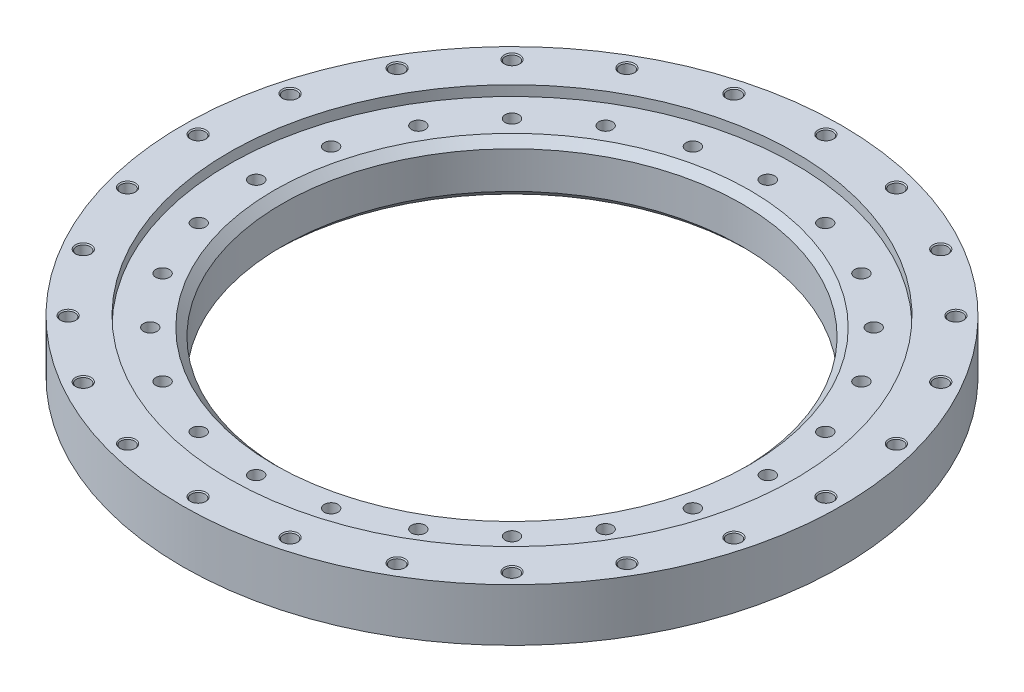
from build123d import *

# Parameters (mm, degrees)
SKETCH1_R                    = 420
BOSS_EXTRUDE1_DEPTH          = 67
SKETCH2_R                    = 360.5
CUT_EXTRUDE1_DEPTH           = 13
SKETCH3_R                    = 360
BOSS_EXTRUDE2_DEPTH          = 13
M20_TAPPED_HOLE1_D           = 17.5
M20_TAPPED_HOLE1_CSINK_D     = 20.05
M20_TAPPED_HOLE1_CSINK_ANGLE = 90
SKETCH6_R                    = 293
CUT_EXTRUDE2_DEPTH           = 598.736564048
CHAMFER1_SIZE                = 10
M20_TAPPED_HOLE2_D           = 17.5
M20_TAPPED_HOLE2_CSINK_D     = 20.05
M20_TAPPED_HOLE2_CSINK_ANGLE = 90


with BuildPart() as part:
    # Sketch1 → Boss-Extrude1 (new body)
    with BuildSketch(Plane(origin=(0, 0, 0), x_dir=(1, 0, 0), z_dir=(0, 1, 0))):
        with Locations(Location((0, 0, 0), (0, 0, 270))):
            Circle(SKETCH1_R)
    extrude(amount=BOSS_EXTRUDE1_DEPTH)

    # Sketch2 → Cut-Extrude1 (cut)
    with BuildSketch(Plane(origin=(0, 67, 0), x_dir=(1, 0, 0), z_dir=(0, 1, 0))):
        with Locations(Location((0, 0, 0), (0, 0, 270))):
            Circle(SKETCH2_R)
    extrude(amount=-CUT_EXTRUDE1_DEPTH, mode=Mode.SUBTRACT)

    # Sketch3 → Boss-Extrude2 (add)
    with BuildSketch(Plane.XZ):
        with Locations(Location((0, 0, 0), (0, 0, 90))):
            Circle(SKETCH3_R)
    extrude(amount=BOSS_EXTRUDE2_DEPTH)

    # M20 Tapped Hole1 (through all)
    with Locations(Plane(origin=(0, 67, 0), x_dir=(1, 0, 0), z_dir=(0, 1, 0))):
        with Locations((-103.527618041, 386.370330516), (0, 400), (103.527618041, 386.370330516), (200, 346.410161514), (282.842712475, 282.842712475), (346.410161514, 200), (386.370330516, 103.527618041), (400, 0), (386.370330516, -103.527618041), (346.410161514, -200), (282.842712475, -282.842712475), (200, -346.410161514), (103.527618041, -386.370330516), (0, -400), (-103.527618041, -386.370330516), (-200, -346.410161514), (-282.842712475, -282.842712475), (-346.410161514, -200), (-386.370330516, -103.527618041), (-400, 0), (-386.370330516, 103.527618041), (-346.410161514, 200), (-282.842712475, 282.842712475), (-200, 346.410161514)):
            CounterSinkHole(M20_TAPPED_HOLE1_D / 2, M20_TAPPED_HOLE1_CSINK_D / 2, counter_sink_angle=M20_TAPPED_HOLE1_CSINK_ANGLE)

    # Sketch6 → Cut-Extrude2 (cut, through all)
    with BuildSketch(Plane(origin=(0, 54, 0), x_dir=(1, 0, 0), z_dir=(0, 1, 0))):
        with Locations(Location((0, 0, 0), (0, 0, 270))):
            Circle(SKETCH6_R)
    extrude(amount=-CUT_EXTRUDE2_DEPTH, mode=Mode.SUBTRACT)

    # Chamfer1
    chamfer1_edges = [part.edges().sort_by_distance(p)[0] for p in [
        (0, -13, -293),
        (0, 54, -293),
    ]]
    chamfer(chamfer1_edges, length=CHAMFER1_SIZE)

    # M20 Tapped Hole2 (through all)
    with Locations(Plane(origin=(0, -13, 0), x_dir=(-1, 0, 0), z_dir=(0, -1, 0))):
        with Locations((-84.375008703, 314.89181937), (0, 326), (84.375008703, 314.89181937), (163, 282.324281634), (230.516810667, 230.516810667), (282.324281634, 163), (314.89181937, 84.375008703), (326, 0), (314.89181937, -84.375008703), (282.324281634, -163), (230.516810667, -230.516810667), (163, -282.324281634), (84.375008703, -314.89181937), (0, -326), (-84.375008703, -314.89181937), (-163, -282.324281634), (-230.516810667, -230.516810667), (-282.324281634, -163), (-314.89181937, -84.375008703), (-326, 0), (-314.89181937, 84.375008703), (-282.324281634, 163), (-230.516810667, 230.516810667), (-163, 282.324281634)):
            CounterSinkHole(M20_TAPPED_HOLE2_D / 2, M20_TAPPED_HOLE2_CSINK_D / 2, counter_sink_angle=M20_TAPPED_HOLE2_CSINK_ANGLE)


solid = part.part
